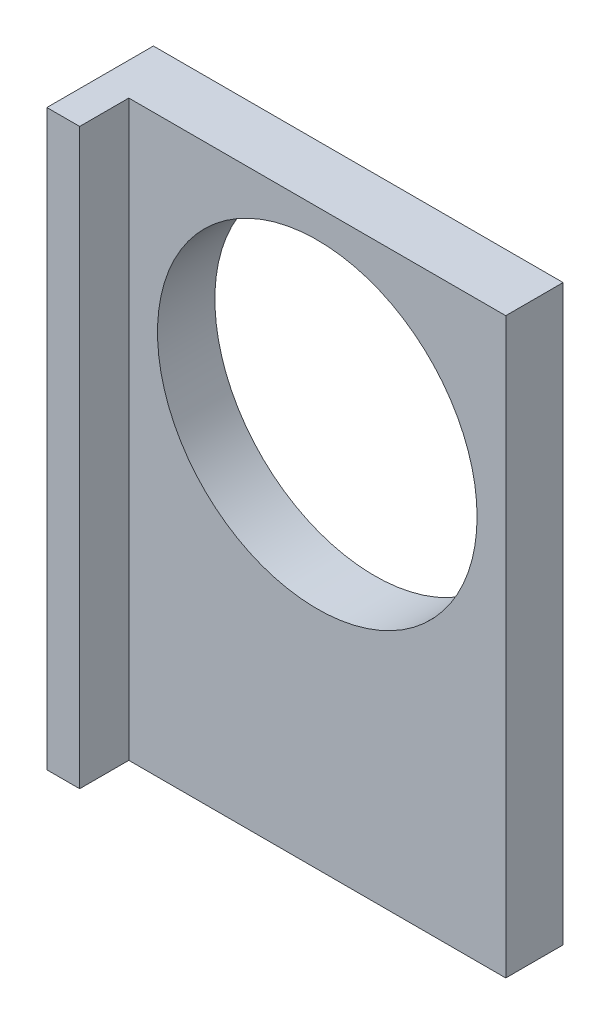
from build123d import *

# Parameters (mm, degrees)
SKETCH_1_W          = 100
SKETCH_1_H          = 140
EXTRUDE_1_DEPTH     = 14
CUT_EXTRUDE_1_REACH = 89.155
SKETCH_2_R          = 39
SKETCH_3_W          = 8
SKETCH_3_H          = 140
EXTRUDE_2_DEPTH     = 12


with BuildPart() as part:
    # 草图1 → 凸台-拉伸1 (new body)
    with BuildSketch(Plane.XY):
        Rectangle(SKETCH_1_W, SKETCH_1_H)
    extrude(amount=EXTRUDE_1_DEPTH)

    # 草图2 → 切除-拉伸1 (cut, up to next)
    with BuildSketch(Plane.XY.offset(14), mode=Mode.PRIVATE) as cut_extrude_1_sk1:
        with Locations((4, 24)):
            Circle(SKETCH_2_R)
    cut_extrude_1_tool1 = extrude(cut_extrude_1_sk1.sketch, amount=-CUT_EXTRUDE_1_REACH, mode=Mode.PRIVATE) & part.part
    add(cut_extrude_1_tool1.solids().sort_by_distance((4, 24, 14))[0], mode=Mode.SUBTRACT)

    # 草图3 → 凸台-拉伸2 (add)
    with BuildSketch(Plane.XY.offset(14)):
        with Locations((-46, 0)):
            Rectangle(SKETCH_3_W, SKETCH_3_H)
    extrude(amount=EXTRUDE_2_DEPTH)


solid = part.part
